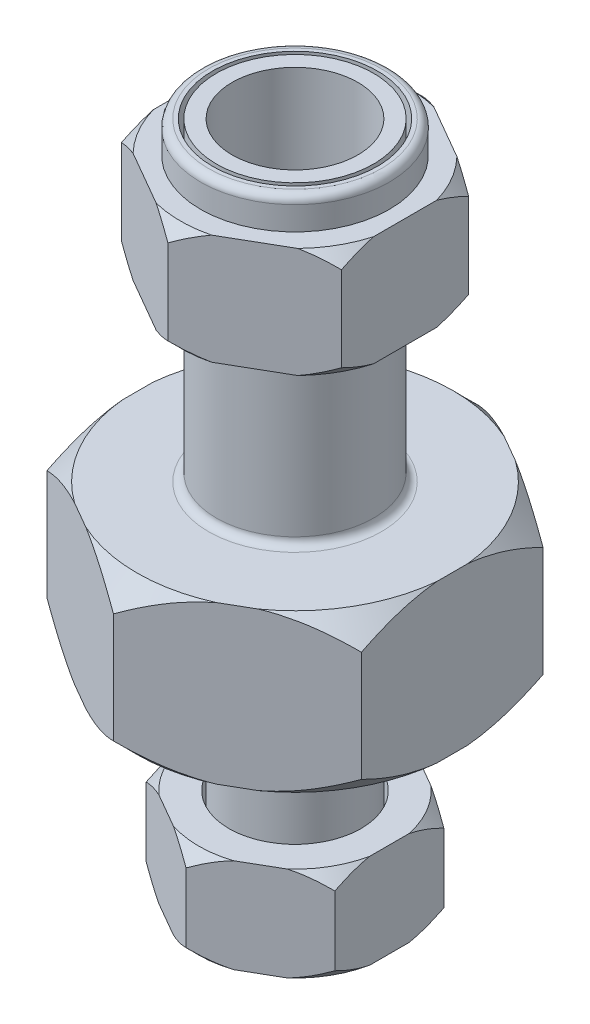
SolidWorks part; units mm, degrees
ref_plane "Front Plane" through (0, 0, 0) normal (0, 0, 1) x (1, 0, 0)
ref_plane "Top Plane" through (0, 0, 0) normal (0, 1, 0) x (1, 0, 0)
ref_plane "Right Plane" through (0, 0, 0) normal (1, 0, 0) x (0, 0, -1)
sketch "Sketch1" plane through (0, 0, 0) normal (0, 1, 0) x (1, 0, 0)
  line L1 (0, -11.547) -> (10, -5.7735)
  line L2 (10, -5.7735) -> (10, 5.7735)
  line L3 (10, 5.7735) -> (0, 11.547)
  line L4 (0, 11.547) -> (-10, 5.7735)
  line L5 (-10, 5.7735) -> (-10, -5.7735)
  line L6 (-10, -5.7735) -> (0, -11.547)
  circle A0 centre (0, 0) radius 10 construction
  dimension "D1" = 20
extrude "Boss-Extrude1" add sketch "Sketch1" along normal blind 10
sketch "Sketch2" plane through (0, 10, 0) normal (0, 1, 0) x (1, 0, 0)
  circle A0 centre (0, 0) radius 5
  dimension "D1" = 10
extrude "Boss-Extrude2" add sketch "Sketch2" along normal blind 20
sketch "Sketch3" plane through (0, 0, 0) normal (0, -1, 0) x (1, 0, 0)
  circle A0 centre (0, 0) radius 4
  dimension "D1" = 8
extrude "Boss-Extrude3" add sketch "Sketch3" along normal blind 14
sketch "Sketch4" plane through (0, -14, 0) normal (0, -1, 0) x (1, 0, 0)
  circle A0 centre (0, 0) radius 3
  dimension "D1" = 6
extrude "Cut-Extrude1" cut sketch "Sketch4" against normal blind 30
sketch "Sketch5" plane through (0, 30, 0) normal (0, 1, 0) x (1, 0, 0)
  circle A0 centre (0, 0) radius 4
  dimension "D1" = 8
extrude "Cut-Extrude2" cut sketch "Sketch5" against normal blind 17
sketch "Sketch6" plane through (0, 30, 0) normal (0, 1, 0) x (1, 0, 0)
  circle A0 centre (0, 0) radius 6
  circle A1 centre (0, 0) radius 5.25
  dimension "D1" = 12
  dimension "D2" = 10.5
extrude "Boss-Extrude4" add sketch "Sketch6" against normal blind 2 separate body
sketch "Sketch7" plane through (0, 28, 0) normal (0, -1, 0) x (1, 0, 0)
  line L1 (0, 8.0829) -> (-7, 4.0415)
  line L2 (-7, 4.0415) -> (-7, -4.0415)
  line L3 (-7, -4.0415) -> (0, -8.0829)
  line L4 (0, -8.0829) -> (7, -4.0415)
  line L5 (7, -4.0415) -> (7, 4.0415)
  line L6 (7, 4.0415) -> (0, 8.0829)
  circle A0 centre (0, 0) radius 5.25 construction
  circle A1 centre (0, 0) radius 5.25
  circle A2 centre (0, 0) radius 7 construction
  dimension "D1" = 14
extrude "Boss-Extrude5" add sketch "Sketch7" along normal blind 7
sketch "Sketch11" plane through (0, -14, 0) normal (0, -1, 0) x (1, 0, 0)
  circle A0 centre (0, 0) radius 4.75
  circle A3 centre (0, 0) radius 4.2
  circle A4 centre (0, 0) radius 4 construction
  dimension "D1" = 9.5
  dimension "D2" = 0.2
extrude "Boss-Extrude6" add sketch "Sketch11" against normal blind 1 separate body
sketch "Sketch12" plane through (0, -13, 0) normal (0, 1, 0) x (1, 0, 0)
  line L1 (0, 6.9282) -> (-6, 3.4641)
  line L2 (-6, 3.4641) -> (-6, -3.4641)
  line L3 (-6, -3.4641) -> (0, -6.9282)
  line L4 (0, -6.9282) -> (6, -3.4641)
  line L5 (6, -3.4641) -> (6, 3.4641)
  line L6 (6, 3.4641) -> (0, 6.9282)
  circle A0 centre (0, 0) radius 4.2 construction
  circle A1 centre (0, 0) radius 4.2
  circle A2 centre (0, 0) radius 6 construction
  dimension "D1" = 12
extrude "Boss-Extrude7" add sketch "Sketch12" along normal blind 6
sketch "Sketch9" plane through (0, 0, 0) normal (1, 0, 0) x (0, 0, -1)
  line L0 (-7.2829, 28) -> (-8.0829, 27.2)
  line L1 (-4.0415, 28) -> (-8.0829, 28) construction
  line L2 (-8.0829, 21) -> (-8.0829, 28) construction
  line L3 (-8.0829, 27.2) -> (-8.0829, 28)
  line L4 (-8.0829, 28) -> (-7.2829, 28)
  line L5 (-8.0829, 24.5) -> (-0.6273, 24.5) construction
  line L6 (-8.0829, 21) -> (-7.2829, 21)
  line L7 (-8.0829, 21.8) -> (-8.0829, 21)
  line L8 (-7.2829, 21) -> (-8.0829, 21.8)
  line L9 (0, 30) -> (0, 37.7244) construction
  line L10 (6, 30) -> (-6, 30) construction
  line L11 (-11.547, 10) -> (-11.547, 8.5)
  line L12 (-11.547, 10) -> (-11.547, 0) construction
  line L13 (-11.547, 8.5) -> (-10.047, 10)
  line L14 (-10.047, 10) -> (-11.547, 10)
  line L15 (-11.547, 5) -> (-4.5484, 5) construction
  line L16 (-10.047, 0) -> (-11.547, 0)
  line L17 (-11.547, 1.5) -> (-10.047, 0)
  line L18 (-11.547, 0) -> (-11.547, 1.5)
  line L19 (-6.9282, -10) -> (3.4609, -10) construction
  line L20 (-6.9282, -7) -> (-6.9282, -13) construction
  line L28 (-6.9282, -7) -> (-6.9282, -7.8)
  line L29 (-6.9282, -7.8) -> (-6.1282, -7)
  line L30 (-6.9282, -7) -> (-3.4641, -7) construction
  line L31 (-6.1282, -7) -> (-6.9282, -7)
  line L32 (-6.1282, -13) -> (-6.9282, -13)
  line L33 (-6.9282, -12.2) -> (-6.1282, -13)
  line L34 (-6.9282, -13) -> (-6.9282, -12.2)
  dimension "D1" = 0.8
  dimension "D2" = 1.5
  dimension "D3" = 0.8
revolve "Cut-Revolve2" cut sketch "Sketch9" angle 360 about L9
fillet "Fillet1" radius 0.5 1 edges at (0, 30, 6)
fillet "Fillet2" radius 0.5 2 edges at (0, 0, -4) (0, 10, 5)
fillet "Fillet3" radius 0.5 1 edges at (0, -14, -4.75)
